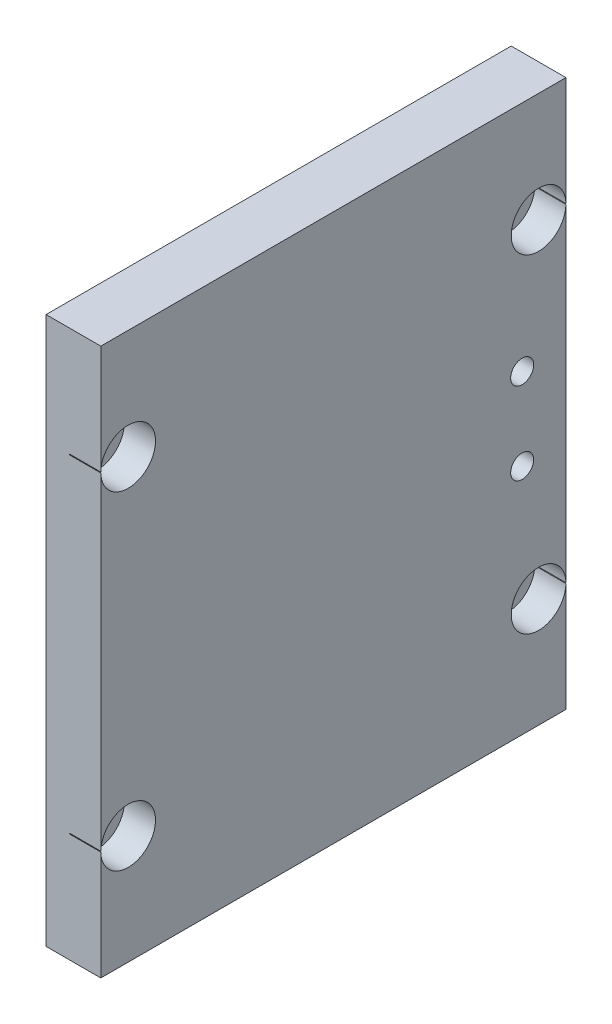
from build123d import *

# Parameters (mm, degrees)
SKETCH_1_W                = 85
SKETCH_1_H                = 100
EXTRUDE_1_DEPTH           = 10
HOLE_WIZARD_1_D           = 5.5
HOLE_WIZARD_1_CBORE_D     = 10.001
HOLE_WIZARD_1_CBORE_DEPTH = 5.7
HOLE_WIZARD_M5_1_D        = 4.2


with BuildPart() as part:
    # 草图1 → 凸台-拉伸1 (new body)
    with BuildSketch(Plane(origin=(0, 0, 0), x_dir=(0, 0, -1), z_dir=(1, 0, 0))):
        Rectangle(SKETCH_1_W, SKETCH_1_H)
    extrude(amount=EXTRUDE_1_DEPTH)

    # 打孔尺寸(%根据)内六角圆柱头螺钉的类型1 (through all)
    with Locations(Plane(origin=(10, 0, 0), x_dir=(0, 0, -1), z_dir=(1, 0, 0))):
        with Locations((-37.5, 30), (-37.5, -30), (37.5, 30), (37.5, -30)):
            CounterBoreHole(HOLE_WIZARD_1_D / 2, HOLE_WIZARD_1_CBORE_D / 2, HOLE_WIZARD_1_CBORE_DEPTH)

    # M5 螺纹孔1 (through all)
    with Locations(Plane(origin=(10, 0, 0), x_dir=(0, 0, -1), z_dir=(1, 0, 0))):
        with Locations((34.5, 7.5), (34.5, -7.5)):
            Hole(HOLE_WIZARD_M5_1_D / 2)


solid = part.part
